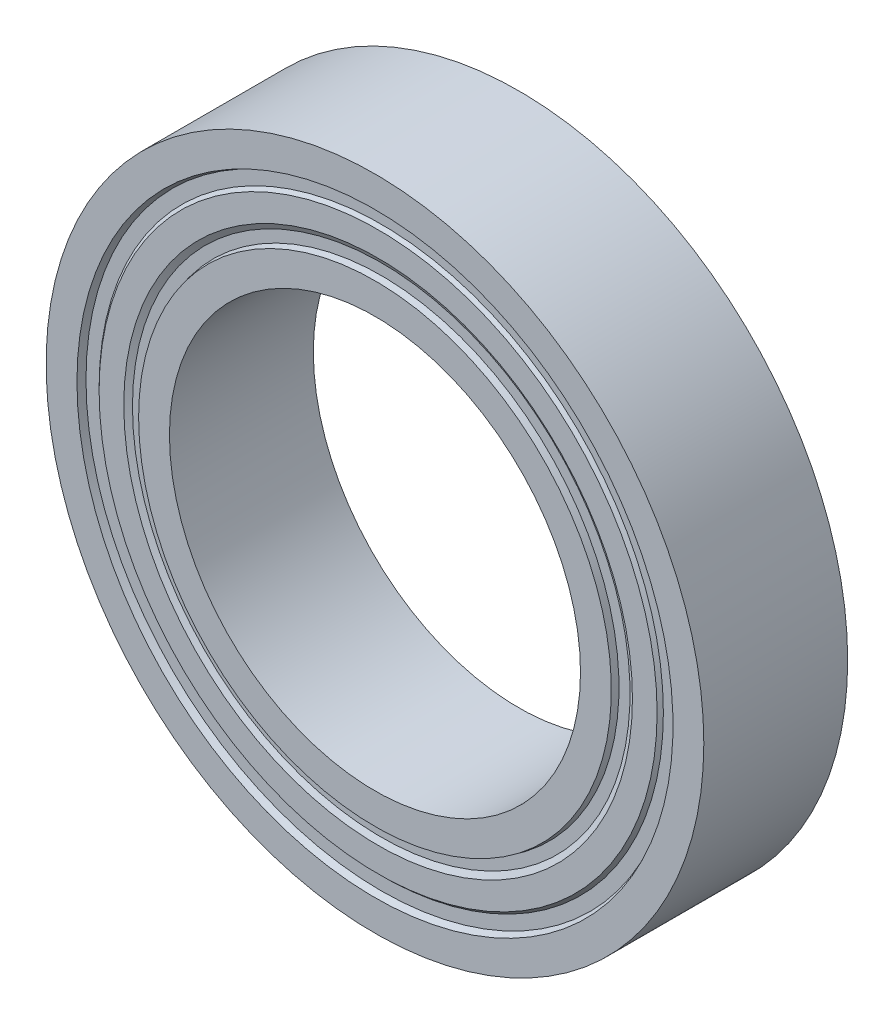
from build123d import *

# Parameters (mm, degrees)
SKETCH1_R           = 16
SKETCH1_R_2         = 10
BOSS_EXTRUDE1_DEPTH = 7


with BuildPart() as part:
    # Sketch1 → Boss-Extrude1 (new body)
    with BuildSketch(Plane.XY):
        Circle(SKETCH1_R)
        Circle(SKETCH1_R_2, mode=Mode.SUBTRACT)
    extrude(amount=BOSS_EXTRUDE1_DEPTH)

    # Sketch3 → Cut-Revolve1 (revolve, cut)
    with BuildSketch(Plane(origin=(0, 0, 0), x_dir=(1, 0, 0), z_dir=(0, 1, 0)), mode=Mode.PRIVATE) as cut_revolve1_sk:
        Polygon((11.5, -7), (11.567254185, -6.694573787), (12.105287665, -6.694573787), (12.374680794, -6.847286894), (13.574680794, -6.847286894), (13.7273939, -6.694573787), (14.365955247, -6.694573787), (14.5, -7), align=None)
    cut_revolve1 = revolve(cut_revolve1_sk.sketch.rotate(Axis((0, 0, 0), (0, 0, 1)), 180), axis=Axis((0, 0, 0), (0, 0, 1)), mode=Mode.SUBTRACT)

    # Mirror1: Cut-Revolve1 across plane
    add(cut_revolve1.mirror(Plane.XY.offset(3.5)), mode=Mode.SUBTRACT)


solid = part.part
